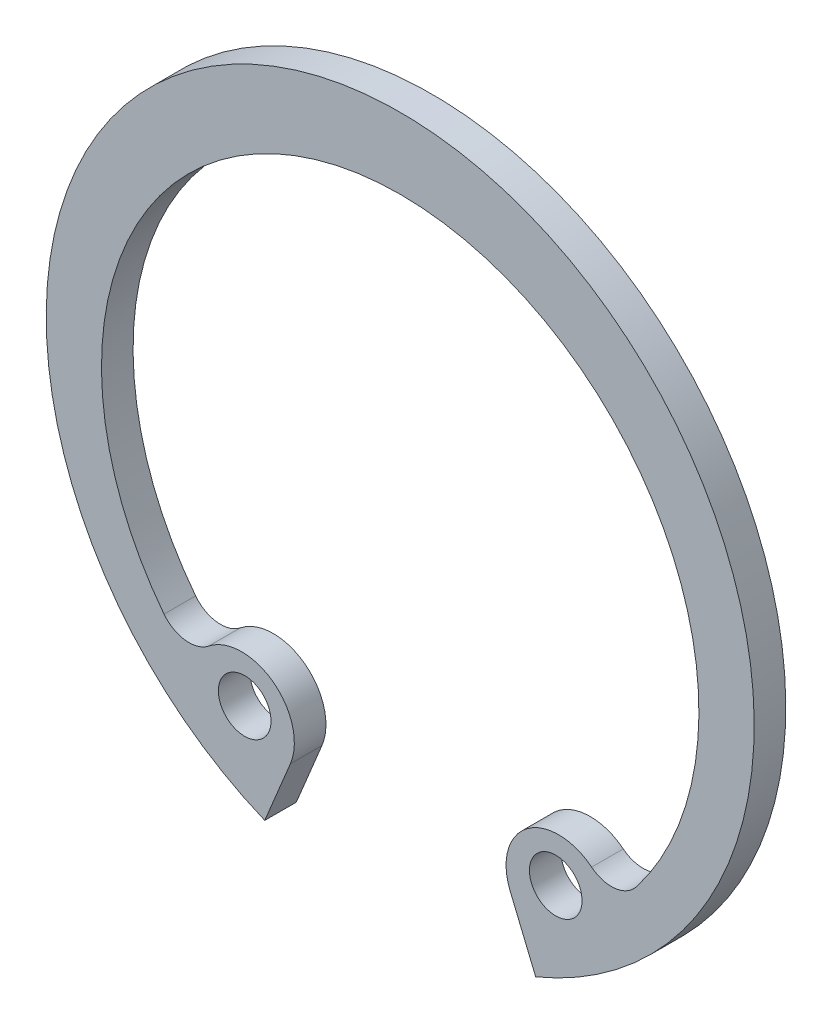
SolidWorks part; units mm, degrees
ref_plane "Front Plane" through (0, 0, 0) normal (0, 0, 1) x (1, 0, 0)
ref_plane "Top Plane" through (0, 0, 0) normal (0, 1, 0) x (1, 0, 0)
ref_plane "Right Plane" through (0, 0, 0) normal (1, 0, 0) x (0, 0, -1)
sketch "Dimension Sketch" plane through (0, 0, 0) normal (0, 0, 1) x (1, 0, 0)
  line L0 (-12.95, 0) -> (12.95, 0) construction
  line L1 (0, 0) -> (-11.215, -6.475) construction
  circle A0 centre (0, 0) radius 12.95
  point P5 (-9.15, 0)
  point P6 (9.6, 0)
  point P7 (2, 0)
  point P8 (10.8, 0)
  point P10 (-2.36, 0)
  point P11 (-0.6, 0)
  point P12 (-4.36, 0)
  point P13 (-10.35, 0)
  point P14 (27.7561, 16.025)
sketch "Sketch1" plane through (0, 0, 0) normal (0, 0, 1) x (1, 0, 0)
  line L0 (0, 13.45) -> (0, -12.4262) construction
  line L1 (-4.1744, -10.0778) -> (-5.1471, -12.4262)
  line L2 (-5.7964, -8.7674) -> (-6.0221, -9.3125) construction
  line L3 (0, 0) -> (-5.1471, -12.4262) construction
  line L4 (4.1744, -10.0778) -> (5.1471, -12.4262)
  arc A0 (5.1471, -12.4262) -> (-5.1471, -12.4262) centre (0, 0) ccw
  arc A1 (8.9726, -7.5508) -> (-8.9726, -7.5508) centre (0, -0.6) ccw
  circle A2 centre (-5.9093, -9.04) radius 1
  arc A3 (-4.1744, -10.0778) -> (-7.2733, -7.7521) centre (-6.0221, -9.3125) ccw
  arc A4 (-7.2733, -7.7521) -> (-8.9726, -7.5508) centre (-8.024, -6.816) cw
  circle A5 centre (5.9093, -9.04) radius 1
  arc A6 (4.1744, -10.0778) -> (7.2733, -7.7521) centre (6.0221, -9.3125) cw
  arc A7 (7.2733, -7.7521) -> (8.9726, -7.5508) centre (8.024, -6.816) ccw
extrude "Base-Extrude" add sketch "Sketch1" along normal blind 1.2
equation "\"D3@Sketch1\" = \"c@Dimension Sketch\""
equation "\"D6@Sketch1\" = \"RR@Dimension Sketch\""
equation "\"D8@Sketch1\" = \"R2@Dimension Sketch\""
equation "\"D7@Sketch1\" = \"R1@Dimension Sketch\""
equation "\"D4@Sketch1\" = \"aa@Dimension Sketch\"/2"
equation "\"D9@Sketch1\" = \"a@Dimension Sketch\""
equation "\"D5@Sketch1\" = \"d1@Dimension Sketch\""
equation "\"D1@Base-Extrude\" = \"s@Dimension Sketch\"/2"
equation "\"D2@Base-Extrude\" = \"D1@Base-Extrude\""
